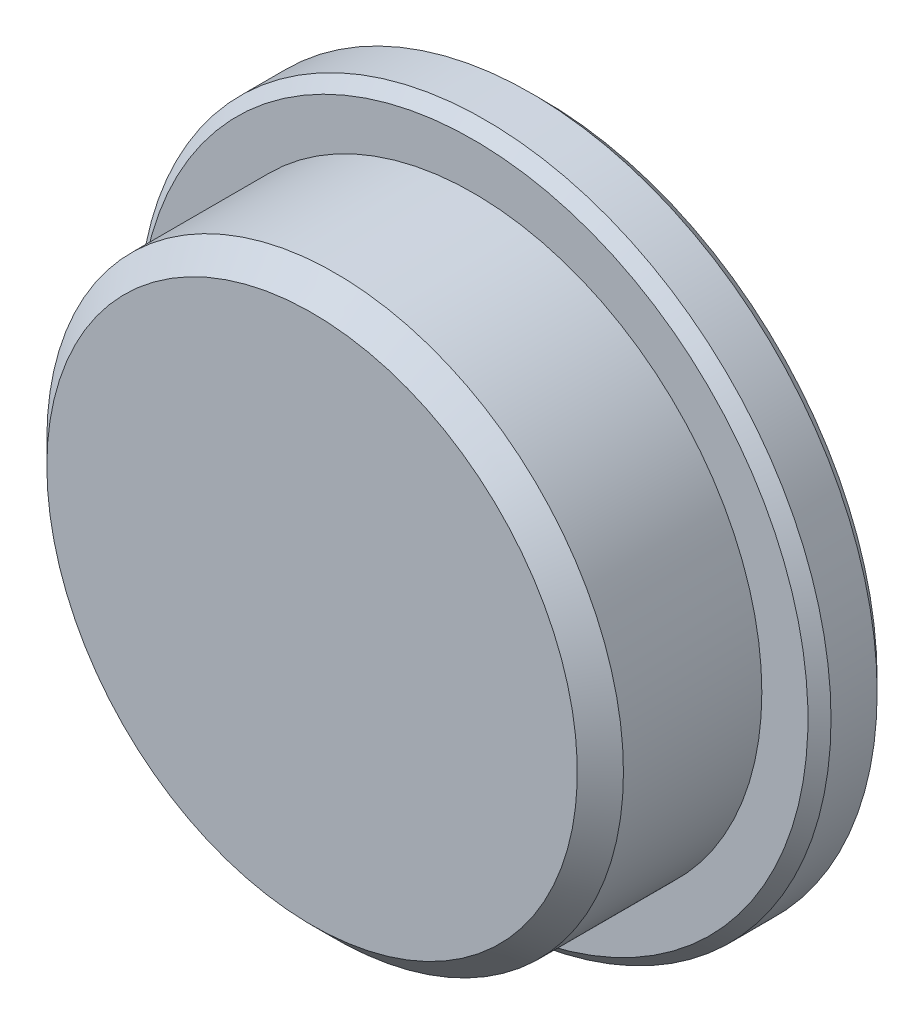
SolidWorks part; units mm, degrees
material "20#"
ref_plane "Front Plane" through (0, 0, 0) normal (0, 0, 1) x (1, 0, 0)
ref_plane "Top Plane" through (0, 0, 0) normal (0, 1, 0) x (1, 0, 0)
ref_plane "Right Plane" through (0, 0, 0) normal (1, 0, 0) x (0, 0, -1)
sketch "Sketch1" plane through (0, 0, 0) normal (1, 0, 0) x (0, 0, -1)
  line L0 (0, 0) -> (10, 0) construction
  line L1 (10, 0) -> (10, 15)
  line L2 (10, 15) -> (7, 15)
  line L3 (7, 15) -> (7, 12.5)
  line L4 (7, 12.5) -> (0, 12.5)
  line L5 (0, 12.5) -> (0, 0)
  line L6 (0, 0) -> (10, 0)
  dimension "D1" = 25
  dimension "D2" = 3
  dimension "D3" = 7
  dimension "D4" = 30
revolve "Revolve1" add sketch "Sketch1" angle 360 about L0
chamfer "Chamfer1" distance 1 angle 45 1 edges at (12.5, 0, 0)
chamfer "Chamfer2" distance 0.5 angle 45 2 edges at (15, 0, -10) (15, 0, -7)
